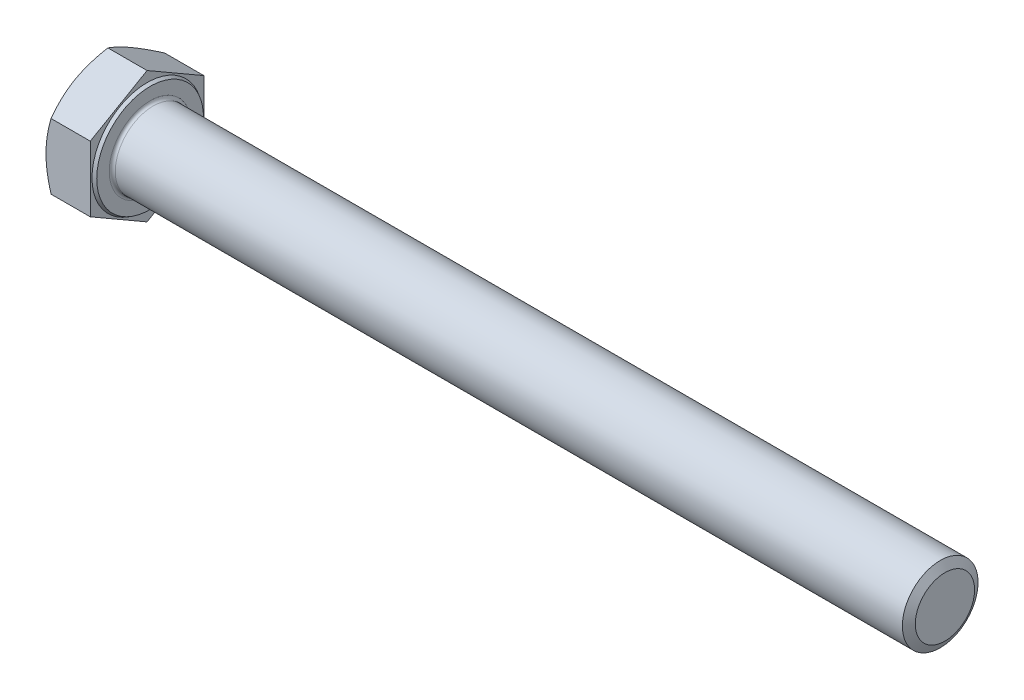
SolidWorks part; units mm, degrees
ref_plane "前视" through (0, 0, 0) normal (0, 0, 1) x (1, 0, 0)
ref_plane "上视" through (0, 0, 0) normal (0, 1, 0) x (1, 0, 0)
ref_plane "右视" through (0, 0, 0) normal (1, 0, 0) x (0, 0, -1)
sketch "草图1" plane through (0, 0, 0) normal (1, 0, 0) x (0, 0, -1)
  line L0 (15, 8.6603) -> (15, -8.6603)
  line L1 (-15, 8.6603) -> (-15, -8.6603)
  line L2 (15, -8.6603) -> (0, -17.3205)
  line L3 (0, -17.3205) -> (-15, -8.6603)
  line L4 (15, 8.6603) -> (0, 17.3205)
  line L5 (0, 17.3205) -> (-15, 8.6603)
  circle A0 centre (0, 0) radius 16.765 construction
  dimension "e" = 33.53
  dimension "s" = 30
  dimension "D2" = 120
  dimension "D3" = 15
  dimension "D4" = 15
  dimension "D5" = 15
extrude "基体-拉伸" add sketch "草图1" along normal blind 12.5
sketch "草图2" plane through (0, 0, 0) normal (0, 0, 1) x (1, 0, 0)
  line L0 (0, 8.6603) -> (0, -8.6603) construction
  line L1 (0, 0) -> (222.5, 0)
  line L2 (0, 0) -> (0, 10)
  line L3 (0, 10) -> (170.5, 10)
  line L4 (222.5, 0) -> (222.5, 7.835)
  line L5 (12.5, 17.3205) -> (12.5, 8.6603) construction
  line L7 (0, 0) -> (242.5, 0) construction
  line L8 (222.5, -7.835) -> (170.5, -10) construction
  line L9 (0, -10) -> (170.5, -10) construction
  line L10 (15, 10) -> (15, 0) construction
  line L11 (170.5, 15.24) -> (170.5, -1.27) construction
  line L12 (12.5, 8.6603) -> (12.5, -8.6603) construction
  line L13 (170.5, 10) -> (222.5, 10)
  line L14 (222.5, 10) -> (222.5, 7.835)
  dimension "l" = 210
  dimension "d" = 20
  dimension "Minor_dia" = 15.67
  dimension "p" = 2.5
  dimension "b" = 52
  dimension "ds" = 20
revolve "凸台-旋转1" add sketch "草图2" angle 360 about L7
cosmetic thread "螺旋线1" parameters "Thread_length"=52, "Thread_minor"=15.67
sketch "草图3" plane through (0, 0, 0) normal (0, 0, 1) x (1, 0, 0)
  line L0 (0, 15) -> (4.2265, 22.3205)
  line L1 (0, 17.3205) -> (0, 8.6603) construction
  line L2 (4.2265, 22.3205) -> (4.2265, 27.3205)
  line L3 (4.2265, 27.3205) -> (-10, 27.3205)
  line L4 (-10, 27.3205) -> (-10, 15)
  line L5 (-10, 15) -> (0, 15)
  line L6 (0, 0) -> (99.06, 0) construction
  line L7 (12.5, 17.3205) -> (0, 17.3205) construction
  dimension "D1" = 15
  dimension "D2" = 5
  dimension "D3" = 10
  dimension "D4" = 5
  dimension "Head_ch_ang" = 30
revolve "切除-旋转1" cut sketch "草图3" angle 360 about L6
sketch "草图4" plane through (0, 0, 0) normal (0, 0, 1) x (1, 0, 0)
  line L0 (12.5, 0) -> (12.5, 14.095) construction
  line L2 (12.5, -10) -> (12.5, 10) construction
  line L3 (12.5, 17.3205) -> (12.5, 8.6603) construction
  line L4 (12.5, 14.095) -> (11.7, 14.5569)
  line L5 (0, 0) -> (95.25, 0) construction
  line L6 (0, 0) -> (242.5, 0) construction
  line L9 (11.7, 14.5569) -> (11.7, 17.3205)
  line L10 (12.5, 17.3205) -> (1.3397, 17.3205) construction
  line L11 (11.7, 17.3205) -> (12.5, 17.3205)
  line L12 (12.5, 17.3205) -> (12.5, 14.095)
  dimension "D1" = 120
  dimension "c" = 0.8
  dimension "dw" = 28.19
revolve "切除-旋转3" cut sketch "草图4" angle 360 about L5
fillet "圆角" radius 0.8 1 edges at (12.5, 0, -10)
sketch "草图6" plane through (0, 0, 0) normal (0, 0, 1) x (1, 0, 0)
  line L0 (0, 0) -> (222.5, 0) construction
  line L1 (222.5, -10) -> (222.5, 10) construction
  line L2 (222.5, 0) -> (222.5, 10) construction
  line L4 (221.25, 10) -> (223.75, 10)
  line L5 (221.25, 10) -> (222.5, 7.8349)
  line L6 (222.5, 7.8349) -> (223.75, 10)
  dimension "D1" = 2.5
revolve "切除-旋转4" cut sketch "草图6" angle 360 about L0
pattern_linear "阵列(线性)1" [suppressed]
